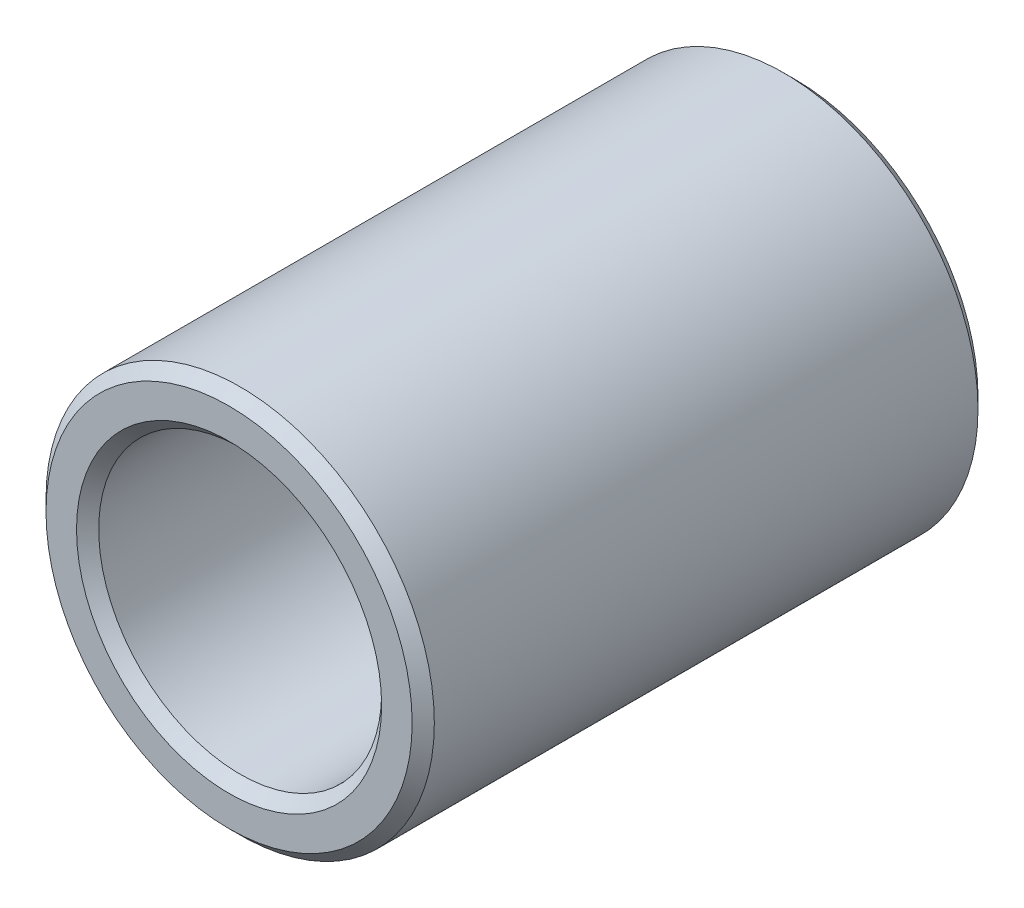
from build123d import *

# Parameters (mm, degrees)
SKETCH_1_R      = 17.5
SKETCH_1_R_2    = 12.75
EXTRUDE_1_DEPTH = 25.5
CHAMFER_1_SIZE  = 1


with BuildPart() as part:
    # 草图1 → 凸台-拉伸1 (new, symmetric)
    with BuildSketch(Plane.XY):
        Circle(SKETCH_1_R)
        Circle(SKETCH_1_R_2, mode=Mode.SUBTRACT)
    extrude(amount=EXTRUDE_1_DEPTH, both=True)

    # 倒角1
    chamfer_1_edges = [part.edges().sort_by_distance(p)[0] for p in [
        (-17.5, 0, -25.5),
        (-17.5, 0, 25.5),
        (-12.75, 0, -25.5),
        (-12.75, 0, 25.5),
    ]]
    chamfer(chamfer_1_edges, length=CHAMFER_1_SIZE)


solid = part.part
